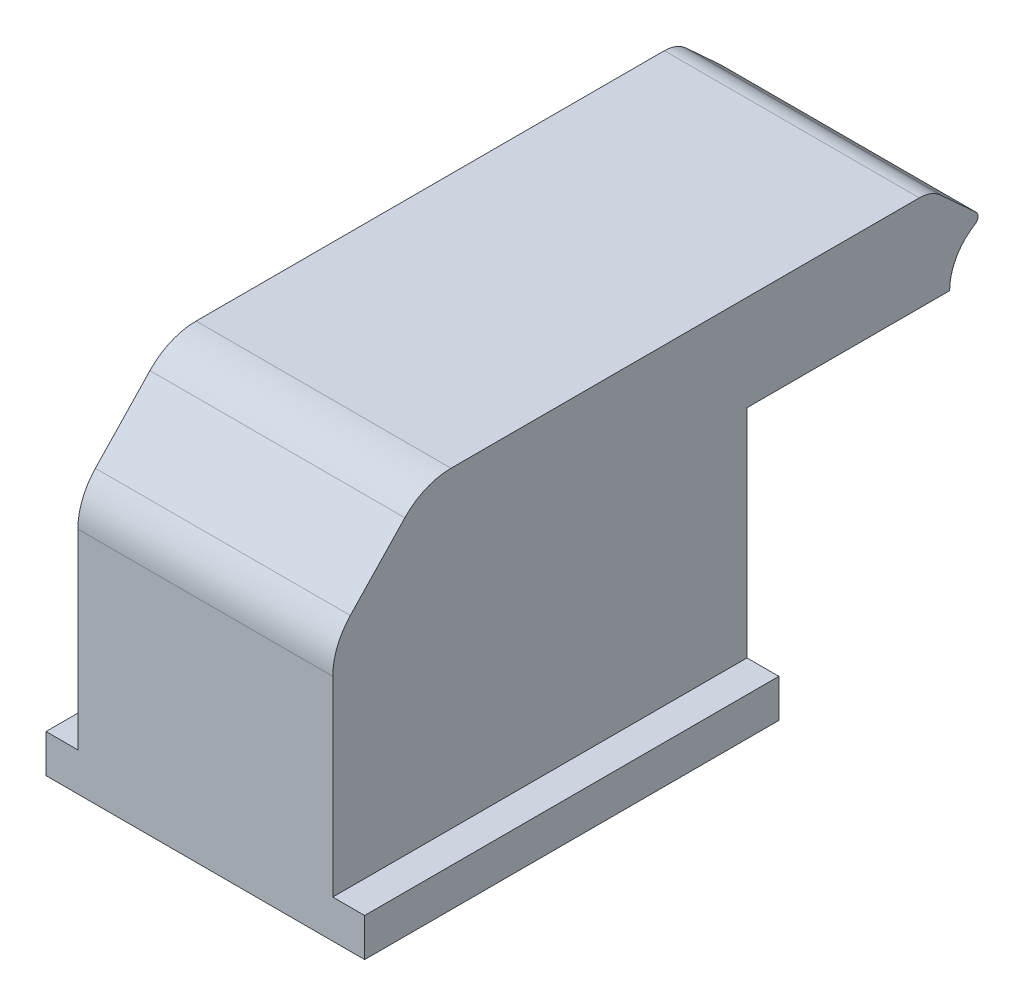
SolidWorks part; units mm, degrees
ref_plane "Front Plane" through (0, 0, 0) normal (0, 0, 1) x (1, 0, 0)
ref_plane "Top Plane" through (0, 0, 0) normal (0, 1, 0) x (1, 0, 0)
ref_plane "Right Plane" through (0, 0, 0) normal (1, 0, 0) x (0, 0, -1)
sketch "Sketch1" plane through (0, 0, 0) normal (0, 1, 0) x (1, 0, 0)
  line L1 (-25, -32.5) -> (25, -32.5)
  line L2 (-25, -32.5) -> (-25, 32.5)
  line L3 (-25, 32.5) -> (25, 32.5)
  line L4 (25, -32.5) -> (25, 32.5)
  line L5 (-25, -32.5) -> (25, 32.5) construction
  line L6 (-25, 32.5) -> (25, -32.5) construction
  point P0 (0, 0)
  dimension "D1" = 50
  dimension "D2" = 65
extrude "Boss-Extrude1" add sketch "Sketch1" along normal blind 6
sketch "Sketch2" plane through (0, 6, 0) normal (0, 1, 0) x (1, 0, 0)
  line L5 (-25, -32.5) -> (25, -32.5) construction
  line L6 (-20, 32.5) -> (20, 32.5)
  line L7 (-20, 32.5) -> (-20, -32.5)
  line L8 (-20, -32.5) -> (20, -32.5)
  line L9 (20, 32.5) -> (20, -32.5)
  line L10 (-20, 32.5) -> (20, -32.5) construction
  line L11 (-20, -32.5) -> (20, 32.5) construction
  point P0 (0, 0)
  dimension "D1" = 40
extrude "Boss-Extrude2" add sketch "Sketch2" along normal blind 34
sketch "Sketch3" plane through (0, 0, -32.5) normal (0, 0, -1) x (-1, 0, 0)
  line L0 (-25, 0) -> (25, 0) construction
  circle A0 centre (0, 25) radius 10.5
  dimension "D1" = 25
  dimension "D2" = 21
extrude "Cut-Extrude1" cut sketch "Sketch3" against normal blind 47
sketch "Sketch4" plane through (0, 0, 0) normal (1, 0, 0) x (0, 0, -1)
  line L0 (-32.5, 40) -> (64.3, 40)
  line L1 (28.3628, 55) -> (-18.236, 55)
  line L6 (-18.236, 55) -> (-32.5, 40)
  line L7 (32.5, 40) -> (32.5, 6) construction
  line L8 (28.3628, 55) -> (59.5352, 55)
  line L9 (62.9201, 53.6801) -> (68.427, 48.6149)
  arc A5 (64.3, 40) -> (68.2663, 47.0225) centre (72.5, 40) cw
  arc A7 (68.2663, 47.0225) -> (68.427, 48.6149) centre (67.75, 47.8789) ccw
  arc A8 (59.5352, 55) -> (62.9201, 53.6801) centre (59.5352, 50) cw
  point P7 (75.2376, 47.7295)
  dimension "D1" = 15
  dimension "D2" = 8.2
  dimension "D3" = 1
  dimension "D4" = 5
  dimension "D5" = 31.8
  dimension "D6" = 100.25
extrude "Boss-Extrude3" add sketch "Sketch4" along normal mid plane 40
fillet "Fillet1" radius 10 2 edges at (0, 55, 18.236) (0, 40, 32.5)
